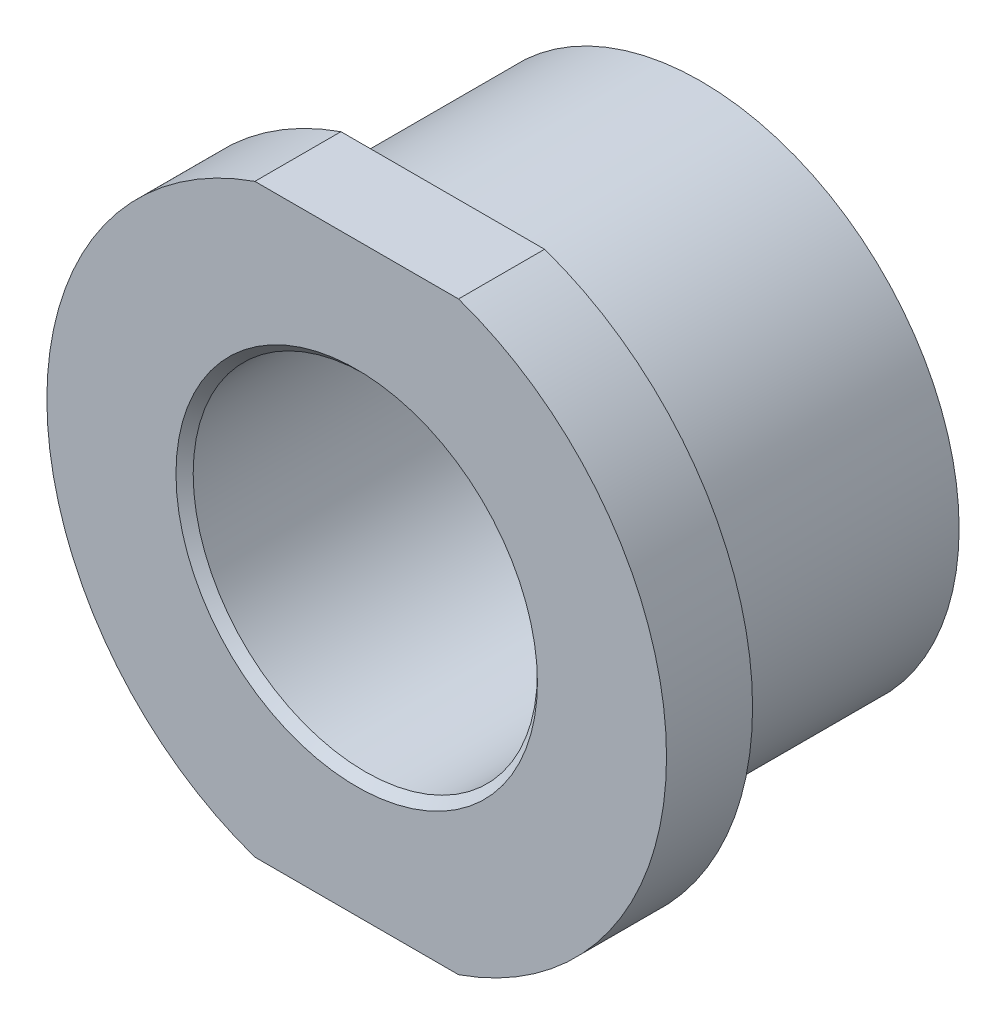
from build123d import *

# Parameters (mm, degrees)
SKETCH1_R           = 15
SKETCH1_R_2         = 10
BOSS_EXTRUDE1_DEPTH = 15
SKETCH2_R           = 10
BOSS_EXTRUDE2_DEPTH = 5
CHAMFER1_SIZE       = 0.5


with BuildPart() as part:
    # Sketch1 → Boss-Extrude1 (new body)
    with BuildSketch(Plane.XY):
        Circle(SKETCH1_R)
        Circle(SKETCH1_R_2, mode=Mode.SUBTRACT)
    extrude(amount=BOSS_EXTRUDE1_DEPTH)

    # Sketch2 → Boss-Extrude2 (add)
    with BuildSketch(Plane.XY.offset(15)):
        with BuildLine():
            Line((-5.916079783, 17), (5.916079783, 17))
            ThreePointArc((5.916079783, 17), (18, 0), (5.916079783, -17))
            Line((5.916079783, -17), (-5.916079783, -17))
            ThreePointArc((-5.916079783, -17), (-18, 0), (-5.916079783, 17))
        make_face()
        Circle(SKETCH2_R, mode=Mode.SUBTRACT)
    extrude(amount=BOSS_EXTRUDE2_DEPTH)

    # Chamfer1
    chamfer1_edges = [part.edges().sort_by_distance(p)[0] for p in [
        (-10, 0, 20),
        (-10, 0, 0),
    ]]
    chamfer(chamfer1_edges, length=CHAMFER1_SIZE)


solid = part.part
